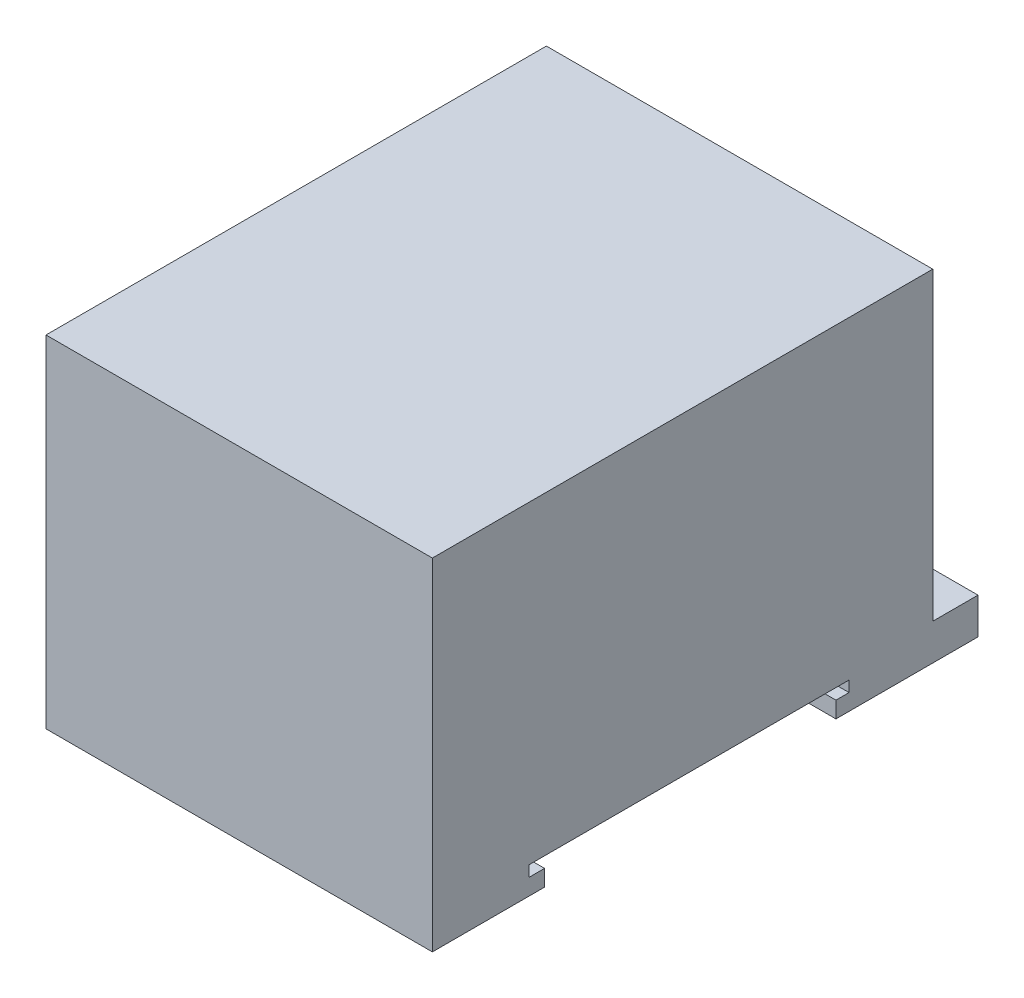
SolidWorks part; units mm, degrees
ref_plane "Front Plane" through (0, 0, 0) normal (0, 0, 1) x (1, 0, 0)
ref_plane "Top Plane" through (0, 0, 0) normal (0, 1, 0) x (1, 0, 0)
ref_plane "Right Plane" through (0, 0, 0) normal (1, 0, 0) x (0, 0, -1)
sketch "Sketch1" plane through (0, 0, 0) normal (0, 1, 0) x (1, 0, 0)
  line L1 (-21.35, -27.65) -> (21.35, -27.65)
  line L2 (-21.35, -27.65) -> (-21.35, 27.65)
  line L3 (-21.35, 27.65) -> (21.35, 27.65)
  line L4 (21.35, -27.65) -> (21.35, 27.65)
  line L5 (-21.35, -27.65) -> (21.35, 27.65) construction
  line L6 (-21.35, 27.65) -> (21.35, -27.65) construction
  point P0 (0, 0)
  dimension "D1" = 55.3
  dimension "D2" = 42.7
extrude "Boss-Extrude1" add sketch "Sketch1" along normal blind 37.7
sketch "Sketch3" plane through (21.35, 0, 0) normal (1, 0, 0) x (0, 0, -1)
  line L0 (-15.25, 0) -> (-15.25, 1.8)
  line L1 (-27.65, 0) -> (27.65, 0) construction
  line L2 (-15.25, 1.8) -> (-16.95, 1.8)
  line L3 (-16.95, 1.8) -> (-16.95, 3)
  line L4 (-16.95, 3) -> (18.3996, 3)
  line L5 (18.3996, 3) -> (18.3996, 1.8)
  line L6 (18.3996, 1.8) -> (16.95, 1.8)
  line L7 (16.95, 1.8) -> (16.95, 0)
  line L8 (-27.65, 37.7) -> (-27.65, 0) construction
  line L9 (-15.25, 0) -> (16.95, 0)
  dimension "D1" = 1.8
  dimension "D2" = 12.4
  dimension "D3" = 1.7
  dimension "D4" = 1.2
  dimension "D5" = 32.2
extrude "Cut-Extrude1" cut sketch "Sketch3" against normal up to next
sketch "Sketch4" plane through (0, 0, 0) normal (0, -1, 0) x (1, 0, 0)
  line L0 (-21.35, 27.65) -> (21.35, 27.65) construction
  line L1 (21.35, -27.65) -> (11.35, -27.65)
  line L2 (21.35, -27.65) -> (21.35, -32.65)
  line L3 (21.35, -32.65) -> (11.35, -32.65)
  line L4 (11.35, -27.65) -> (11.35, -32.65)
  dimension "D1" = 60.3
  dimension "D2" = 10
extrude "Boss-Extrude2" add sketch "Sketch4" against normal blind 4
